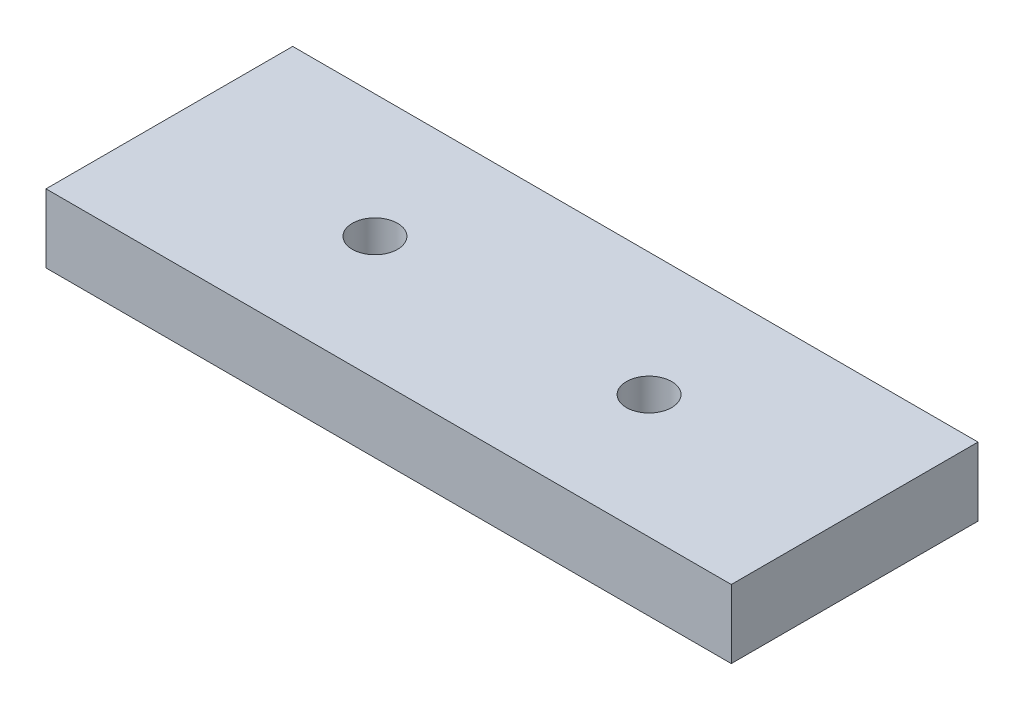
from build123d import *

# Parameters (mm, degrees)
EXTRUDE_1_DEPTH        = 2.5
HOLE_WIZARD_M4_1_D     = 3.3
HOLE_WIZARD_M4_1_DEPTH = 10.1
HOLE_WIZARD_M4_1_TIP   = 0.991420021


with BuildPart() as part:
    # 草图1 → 凸台-拉伸1 (new, symmetric)
    with BuildSketch(Plane(origin=(0, 0, 0), x_dir=(1, 0, 0), z_dir=(0, 1, 0))):
        Polygon((0, 0), (0, -9), (50, -9), (50, 9), (0, 9), align=None)
    extrude(amount=EXTRUDE_1_DEPTH, both=True)

    # M4 螺纹孔1
    with Locations(Plane(origin=(0, 2.5, 0), x_dir=(1, 0, 0), z_dir=(0, 1, 0))):
        with Locations((15, 0), (35, 0)):
            Hole(HOLE_WIZARD_M4_1_D / 2, depth=HOLE_WIZARD_M4_1_DEPTH)
            with Locations((0, 0, -(HOLE_WIZARD_M4_1_DEPTH + HOLE_WIZARD_M4_1_TIP / 2))):  # 118° drill point
                Cone(0, HOLE_WIZARD_M4_1_D / 2, HOLE_WIZARD_M4_1_TIP, mode=Mode.SUBTRACT)


solid = part.part
